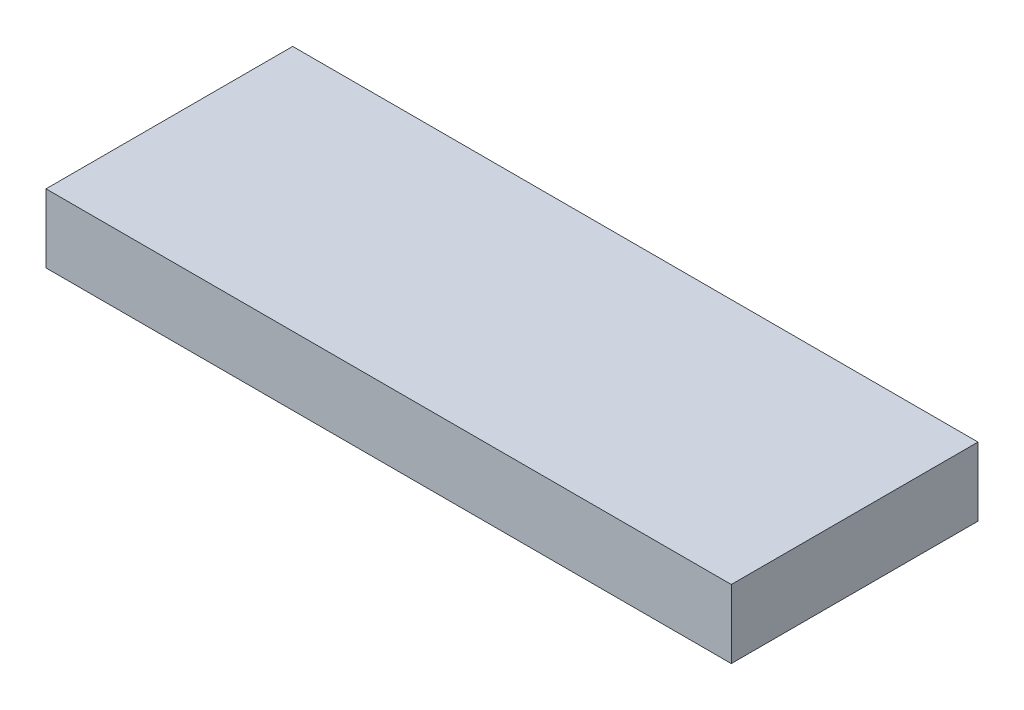
SolidWorks part; units mm, degrees
ref_plane "前视基准面" through (0, 0, 0) normal (0, 0, 1) x (1, 0, 0)
ref_plane "上视基准面" through (0, 0, 0) normal (0, 1, 0) x (1, 0, 0)
ref_plane "右视基准面" through (0, 0, 0) normal (1, 0, 0) x (0, 0, -1)
sketch "草图1" plane through (0, 0, 0) normal (0, 1, 0) x (1, 0, 0)
  line L1 (-250, 90) -> (250, 90)
  line L2 (-250, 90) -> (-250, -90)
  line L3 (-250, -90) -> (250, -90)
  line L4 (250, 90) -> (250, -90)
  line L5 (-250, 90) -> (250, -90) construction
  line L6 (-250, -90) -> (250, 90) construction
  point P0 (0, 0)
  dimension "D1" = 500
  dimension "D2" = 180
extrude "凸台-拉伸1" add sketch "草图1" along normal blind 50
